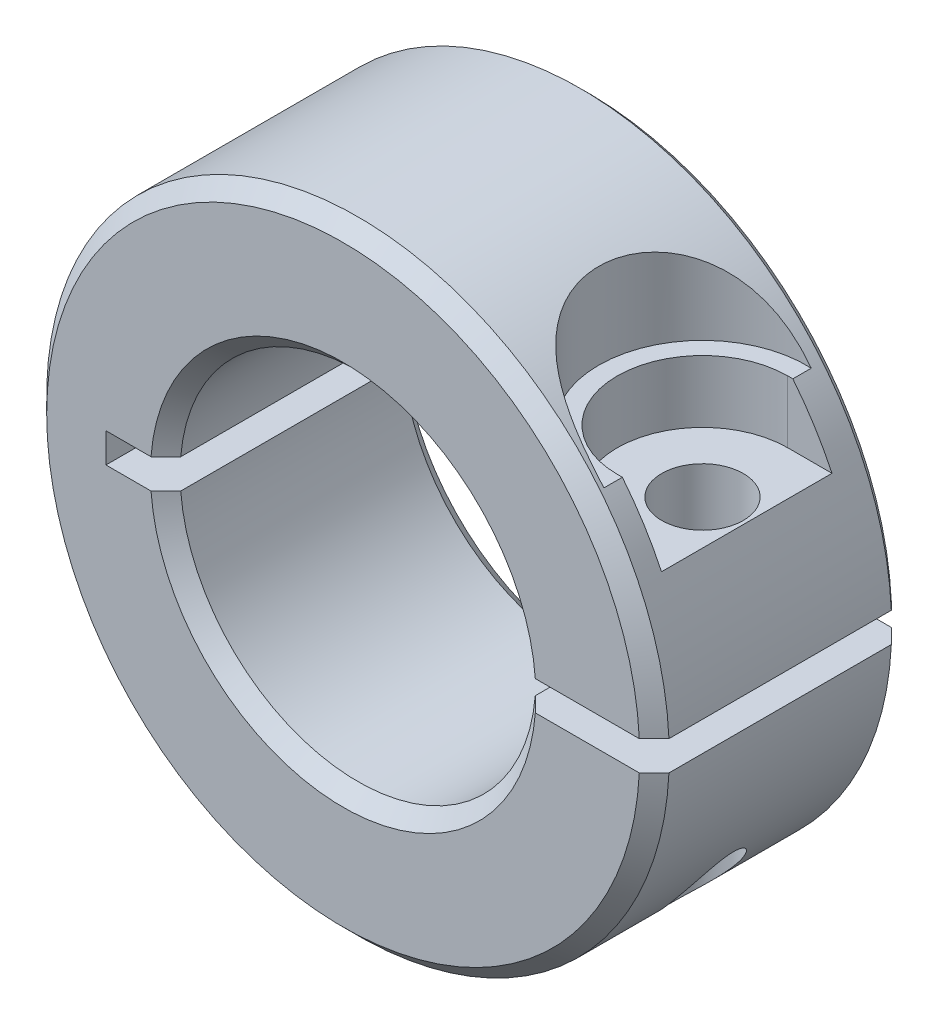
from build123d import *

# Parameters (mm, degrees)
SKETCH2_R             = 21
SKETCH2_R_2           = 12
BOSS_EXTRUDE2_DEPTH   = 17
CHAMFER1_SIZE         = 1
SKETCH3_W             = 46.185652856
SKETCH3_H             = 2
CUT_EXTRUDE1_DEPTH    = 35.219877265
SKETCH5_R             = 2.75
CUT_EXTRUDE3_DEPTH    = 30
CUT_EXTRUDE4_START    = -8
CUT_EXTRUDE4_DEPTH    = 30
M5_TAPPED_HOLE1_D     = 4.2
SKETCH9_W             = 59.171214414
SKETCH9_H             = 29.501144874
CUT_EXTRUDE5_DEPTH    = 0.5
M4_TAPPED_HOLE1_D     = 3.3
M4_TAPPED_HOLE1_DEPTH = 10.1
M4_TAPPED_HOLE1_TIP   = 0.991420021
SKETCH13_R            = 7
CUT_EXTRUDE7_DEPTH    = 17


with BuildPart() as part:
    # Sketch2 → Boss-Extrude2 (new body)
    with BuildSketch(Plane.XY):
        Circle(SKETCH2_R)
        Circle(SKETCH2_R_2, mode=Mode.SUBTRACT)
    extrude(amount=BOSS_EXTRUDE2_DEPTH)

    # Chamfer1
    chamfer1_edges = [part.edges().sort_by_distance(p)[0] for p in [
        (-21, 0, 0),
        (-21, 0, 17),
        (-12, 0, 0),
        (-12, 0, 17),
    ]]
    chamfer(chamfer1_edges, length=CHAMFER1_SIZE)

    # Sketch3 → Cut-Extrude1 (cut, through all)
    with BuildSketch(Plane.XY.offset(17)):
        with Locations((7.092826428, 0)):
            Rectangle(SKETCH3_W, SKETCH3_H)
    extrude(amount=-CUT_EXTRUDE1_DEPTH, mode=Mode.SUBTRACT)

    # Sketch5 → Cut-Extrude3 (cut)
    with BuildSketch(Plane.XZ.offset(-1)):
        with Locations(Location((15.988088482, 8.75, 0), (0, 0, 270))):
            Circle(SKETCH5_R)
    extrude(amount=-CUT_EXTRUDE3_DEPTH, mode=Mode.SUBTRACT)

    # Sketch6 → Cut-Extrude4 (cut)
    with BuildSketch(Plane.XZ.offset(-1).offset(CUT_EXTRUDE4_START)):
        with BuildLine():
            Line((15.988088482, 14.5), (20.976176963, 14.5))
            Line((20.976176963, 14.5), (20.976176963, 3))
            Line((20.976176963, 3), (15.988088482, 3))
            ThreePointArc((15.988088482, 3), (10.238088482, 8.75), (15.988088482, 14.5))
        make_face()
    extrude(amount=-CUT_EXTRUDE4_DEPTH, mode=Mode.SUBTRACT)

    # M5 Tapped Hole1 (through all)
    with Locations(Plane(origin=(0, -1, 0), x_dir=(1, 0, 0), z_dir=(0, 1, 0))):
        with Locations((15.988088482, -8.75)):
            Hole(M5_TAPPED_HOLE1_D / 2)

    # Sketch9 → Cut-Extrude5 (cut)
    with BuildSketch(Plane(origin=(0, 0, 0), x_dir=(-1, 0, 0), z_dir=(0, 0, -1))):
        with Locations((-1.080150951, 14.750572437)):
            Rectangle(SKETCH9_W, SKETCH9_H)
    extrude(amount=-CUT_EXTRUDE5_DEPTH, mode=Mode.SUBTRACT)

    # M4 Tapped Hole1
    with Locations(Plane(origin=(0, 0, 0), x_dir=(-1, 0, 0), z_dir=(0, 0, -1))):
        with Locations((16.444620864, -5.985352508), (-8.75, -15.155444566), (5.985352508, -16.444620864)):
            Hole(M4_TAPPED_HOLE1_D / 2, depth=M4_TAPPED_HOLE1_DEPTH)
            with Locations((0, 0, -(M4_TAPPED_HOLE1_DEPTH + M4_TAPPED_HOLE1_TIP / 2))):  # 118° drill point
                Cone(0, M4_TAPPED_HOLE1_D / 2, M4_TAPPED_HOLE1_TIP, mode=Mode.SUBTRACT)

    # Sketch13 → Cut-Extrude7 (cut)
    with BuildSketch(Plane(origin=(0, 13.2, 0), x_dir=(1, 0, 0), z_dir=(0, 1, 0))):
        with Locations((15.988088482, -8.75)):
            Circle(SKETCH13_R)
    extrude(amount=CUT_EXTRUDE7_DEPTH, mode=Mode.SUBTRACT)


solid = part.part
